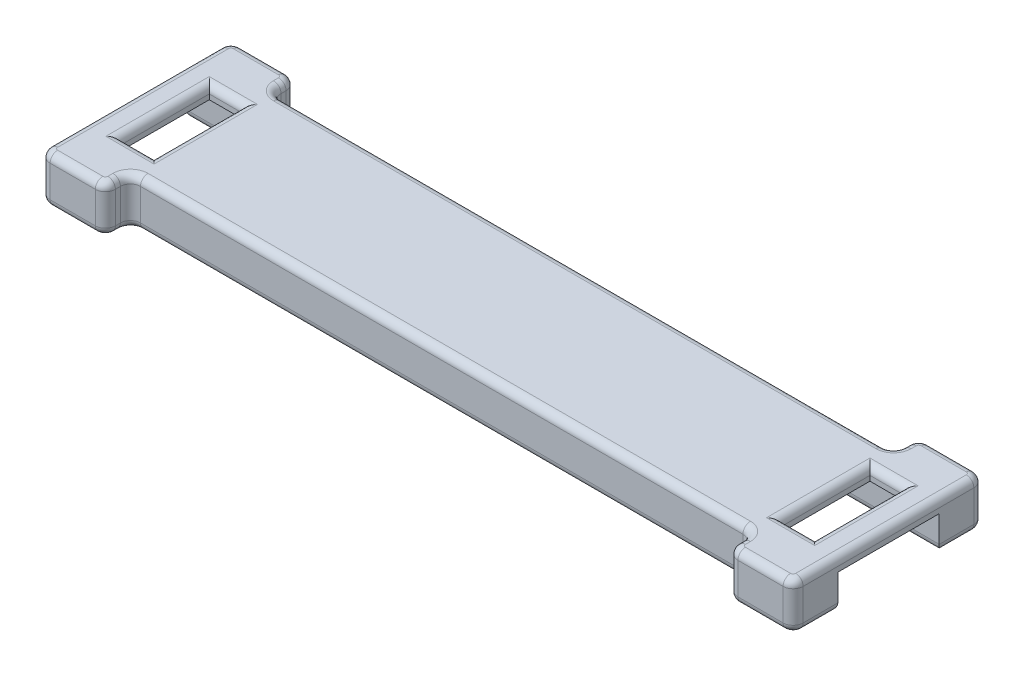
from build123d import *

# Parameters (mm, degrees)
SKETCH_1_W          = 6.6
SKETCH_1_H          = 17.6
EXTRUDE_1_DEPTH     = 9.3
SKETCH_2_W          = 20.2
SKETCH_2_H          = 13.6
CUT_EXTRUDE_1_DEPTH = 20
FILLET_2_R          = 1.5


with BuildPart() as part:
    # 草图1 → 凸台-拉伸1 (new body)
    with BuildSketch(Plane(origin=(0, 0, 0), x_dir=(1, 0, 0), z_dir=(0, 1, 0))):
        with BuildLine():
            Line((-62, 16), (-62, 17))
            ThreePointArc((-62, 17), (-62.585786438, 18.414213562), (-64, 19))
            Line((-64, 19), (-73, 19))
            ThreePointArc((-73, 19), (-74.414213562, 18.414213562), (-75, 17))
            Line((-75, 17), (-75, -17))
            ThreePointArc((-75, -17), (-74.414213562, -18.414213562), (-73, -19))
            Line((-73, -19), (-64, -19))
            ThreePointArc((-64, -19), (-62.585786438, -18.414213562), (-62, -17))
            Line((-62, -17), (-62, -16))
            ThreePointArc((-62, -16), (-61.414213562, -14.585786438), (-60, -14))
            Line((-60, -14), (60, -14))
            ThreePointArc((60, -14), (61.414213562, -14.585786438), (62, -16))
            Line((62, -16), (62, -17))
            ThreePointArc((62, -17), (62.585786438, -18.414213562), (64, -19))
            Line((64, -19), (73, -19))
            ThreePointArc((73, -19), (74.414213562, -18.414213562), (75, -17))
            Line((75, -17), (75, 17))
            ThreePointArc((75, 17), (74.414213562, 18.414213562), (73, 19))
            Line((73, 19), (64, 19))
            ThreePointArc((64, 19), (62.585786438, 18.414213562), (62, 17))
            Line((62, 17), (62, 16))
            ThreePointArc((62, 16), (61.414213562, 14.585786438), (60, 14))
            Line((60, 14), (-60, 14))
            ThreePointArc((-60, 14), (-61.414213562, 14.585786438), (-62, 16))
        make_face()
        with Locations((65.8, 0)):
            Rectangle(SKETCH_1_W, SKETCH_1_H, mode=Mode.SUBTRACT)
        with Locations((-65.8, 0)):
            Rectangle(SKETCH_1_W, SKETCH_1_H, mode=Mode.SUBTRACT)
    extrude(amount=EXTRUDE_1_DEPTH)

    # 草图2 → 切除-拉伸1 (cut)
    with BuildSketch(Plane(origin=(75, 0, 0), x_dir=(0, 0, -1), z_dir=(1, 0, 0))):
        Rectangle(SKETCH_2_W, SKETCH_2_H)
    cut_extrude_1 = extrude(amount=-CUT_EXTRUDE_1_DEPTH, mode=Mode.SUBTRACT)

    # 镜向1: 切除-拉伸1 across plane
    add(cut_extrude_1.mirror(Plane(origin=(0, 0, 0), x_dir=(0, 0, 1), z_dir=(1, 0, 0))), mode=Mode.SUBTRACT)

    # 圆角2
    fillet_2_edges = [part.edges().sort_by_distance(p)[0] for p in [
        (74.414213562, 9.3, 18.414213562),
        (55, 0, 0),
        (65, 0, -10.1),
        (65, 0, 10.1),
        (-75, 0, 13.55),
        (-55, 0, 0),
        (-65, 0, -10.1),
        (75, 9.3, 0),
        (-65, 0, 10.1),
        (74.414213562, 9.3, -18.414213562),
        (68.5, 9.3, -19),
        (62, 0, 16.5),
        (61.414213562, 0, 14.585786438),
        (0, 0, 14),
        (-61.414213562, 0, 14.585786438),
        (62.585786438, 9.3, -18.414213562),
        (-62, 0, 16.5),
        (-62.585786438, 0, 18.414213562),
        (-68.5, 0, 19),
        (-74.414213562, 0, 18.414213562),
        (-75, 0, -13.55),
        (-74.414213562, 0, -18.414213562),
        (-68.5, 0, -19),
        (-62.585786438, 0, -18.414213562),
        (62, 9.3, -16.5),
        (-62, 0, -16.5),
        (-61.414213562, 0, -14.585786438),
        (0, 0, -14),
        (61.414213562, 0, -14.585786438),
        (62, 0, -16.5),
        (62.585786438, 0, -18.414213562),
        (68.5, 0, -19),
        (61.414213562, 9.3, -14.585786438),
        (74.414213562, 0, -18.414213562),
        (75, 0, 13.55),
        (74.414213562, 0, 18.414213562),
        (68.5, 0, 19),
        (62.585786438, 0, 18.414213562),
        (0, 9.3, -14),
        (-61.414213562, 9.3, -14.585786438),
        (-62, 9.3, -16.5),
        (62.585786438, 9.3, 18.414213562),
        (-62.585786438, 9.3, -18.414213562),
        (-68.5, 9.3, -19),
        (-74.414213562, 9.3, -18.414213562),
        (-75, 9.3, 0),
        (-74.414213562, 9.3, 18.414213562),
        (-68.5, 9.3, 19),
        (-62.585786438, 9.3, 18.414213562),
        (69.1, 9.3, 0),
        (65.8, 9.3, -8.8),
        (-62, 9.3, 16.5),
        (62.5, 9.3, 0),
        (65.8, 9.3, 8.8),
        (-61.414213562, 9.3, 14.585786438),
        (0, 9.3, 14),
        (68.5, 9.3, 19),
        (61.414213562, 9.3, 14.585786438),
        (62, 9.3, 16.5),
        (-62.5, 9.3, 0),
        (-65.8, 9.3, -8.8),
        (-69.1, 9.3, 0),
        (-65.8, 9.3, 8.8),
        (75, 0, -13.55),
    ]]
    fillet(fillet_2_edges, radius=FILLET_2_R)


solid = part.part
